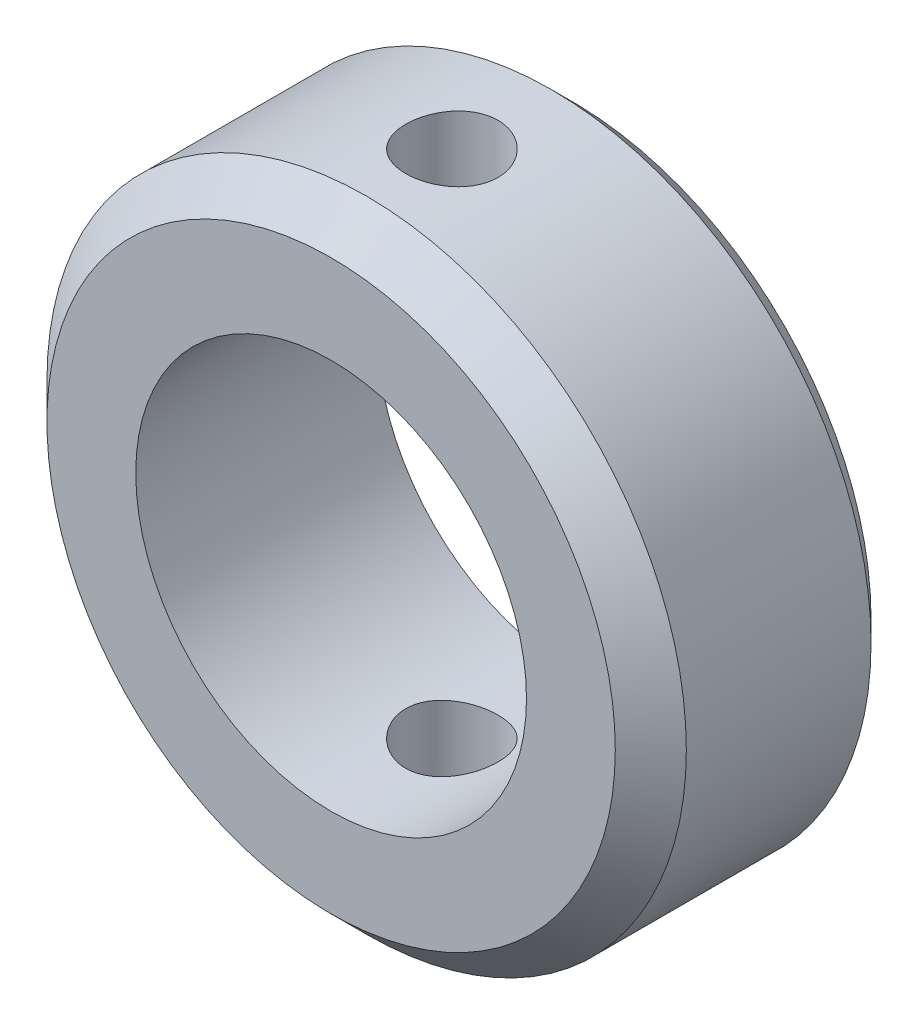
SolidWorks part; units mm, degrees
ref_plane "Front Plane" through (0, 0, 0) normal (0, 0, 1) x (1, 0, 0)
ref_plane "Top Plane" through (0, 0, 0) normal (0, 1, 0) x (1, 0, 0)
ref_plane "Right Plane" through (0, 0, 0) normal (1, 0, 0) x (0, 0, -1)
sketch "Sketch1" plane through (0, 0, 0) normal (0, 0, 1) x (1, 0, 0)
  circle A0 centre (0, 0) radius 27.5
  circle A1 centre (0, 0) radius 45
  dimension "D1" = 55
  dimension "D2" = 90
extrude "Boss-Extrude1" add sketch "Sketch1" along normal blind 34
sketch "Sketch3" plane through (0, 0, 0) normal (0, 1, 0) x (1, 0, 0)
  line L0 (-27.5, -34) -> (27.5, -34) construction
  line L1 (0, 0) -> (0, -40.3636) construction
  circle A0 centre (0, -17) radius 6.5
  dimension "D2" = 13
  dimension "D1" = 17
extrude "Cut-Extrude1" cut sketch "Sketch3" against normal through all and the other way through all
chamfer "Chamfer1" distance 5 angle 45 1 edges at (45, 0, 34)
chamfer "Chamfer2" distance 3 angle 45 1 edges at (45, 0, 0)
